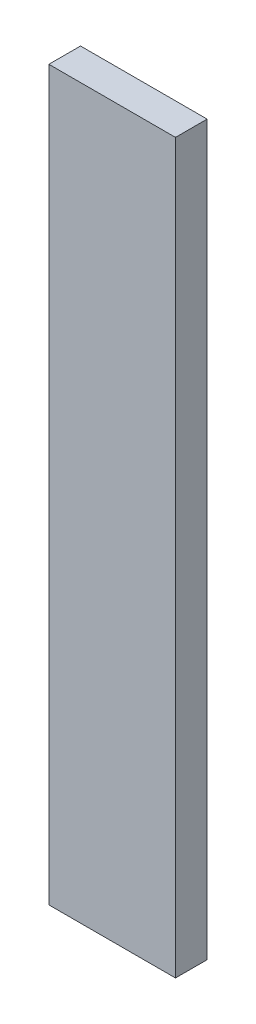
from build123d import *

# Parameters (mm, degrees)
SKETCH1_W           = 80
SKETCH1_H           = 460
BOSS_EXTRUDE1_DEPTH = 20


with BuildPart() as part:
    # Sketch1 → Boss-Extrude1 (new body)
    with BuildSketch(Plane.XY):
        Rectangle(SKETCH1_W, SKETCH1_H)
    extrude(amount=BOSS_EXTRUDE1_DEPTH)


solid = part.part
